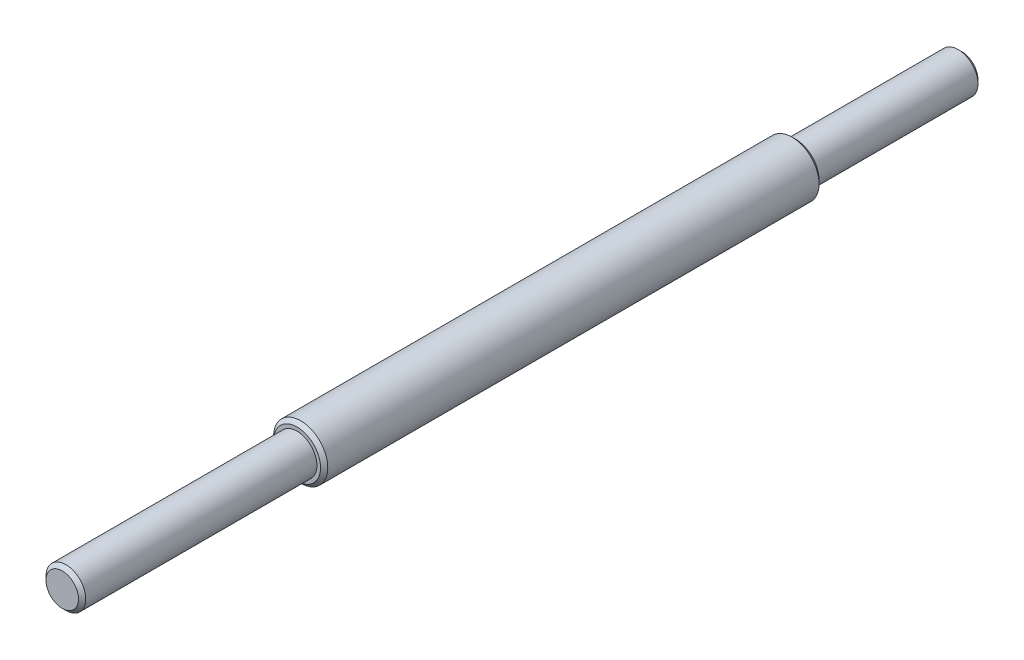
SolidWorks part; units mm, degrees
ref_plane "Front Plane" through (0, 0, 0) normal (0, 0, 1) x (1, 0, 0)
ref_plane "Top Plane" through (0, 0, 0) normal (0, 1, 0) x (1, 0, 0)
ref_plane "Right Plane" through (0, 0, 0) normal (1, 0, 0) x (0, 0, -1)
sketch "Sketch1" plane through (0, 0, 0) normal (0, 0, 1) x (1, 0, 0)
  circle A0 centre (0, 0) radius 7.5
  dimension "D1" = 15
extrude "Boss-Extrude1" add sketch "Sketch1" along normal blind 138
sketch "Sketch2" plane through (0, 0, 138) normal (0, 0, 1) x (1, 0, 0)
  circle A0 centre (0, 0) radius 5.5
  dimension "D1" = 11
extrude "Boss-Extrude2" add sketch "Sketch2" along normal blind 20
sketch "Sketch3" plane through (0, 0, 158) normal (0, 0, 1) x (1, 0, 0)
  circle A0 centre (0, 0) radius 5.5
  dimension "D1" = 11
extrude "Boss-Extrude3" add sketch "Sketch3" along normal blind 45
chamfer "Chamfer1" distance 1 angle 45 3 edges at (5.5, 0, 203) (7.5, 0, 0) (7.5, 0, 138)
sketch "Sketch4" plane through (0, 0, 0) normal (0, 0, -1) x (-1, 0, 0)
  circle A0 centre (0, 0) radius 5.5
  dimension "D1" = 11
extrude "Boss-Extrude4" add sketch "Sketch4" along normal blind 46
chamfer "Chamfer2" distance 1 angle 45 1 edges at (-5.5, 0, -46)
